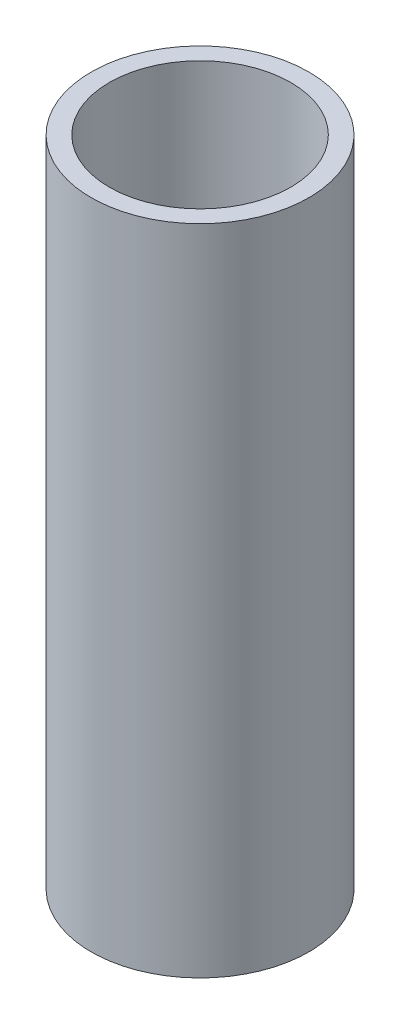
from build123d import *

# Parameters (mm, degrees)
SKETCH_1_R           = 30
SKETCH_1_R_2         = 25
BOSS_EXTRUDE_1_DEPTH = 90


with BuildPart() as part:
    # Sketch 1 → Boss-Extrude 1 (new, symmetric)
    with BuildSketch(Plane(origin=(0, 0, 0), x_dir=(1, 0, 0), z_dir=(0, 1, 0))):
        with Locations(Location((0, 0, 0), (0, 0, 90))):
            Circle(SKETCH_1_R)
        with Locations(Location((0, 0, 0), (0, 0, 90))):
            Circle(SKETCH_1_R_2, mode=Mode.SUBTRACT)
    extrude(amount=BOSS_EXTRUDE_1_DEPTH, both=True)


solid = part.part
